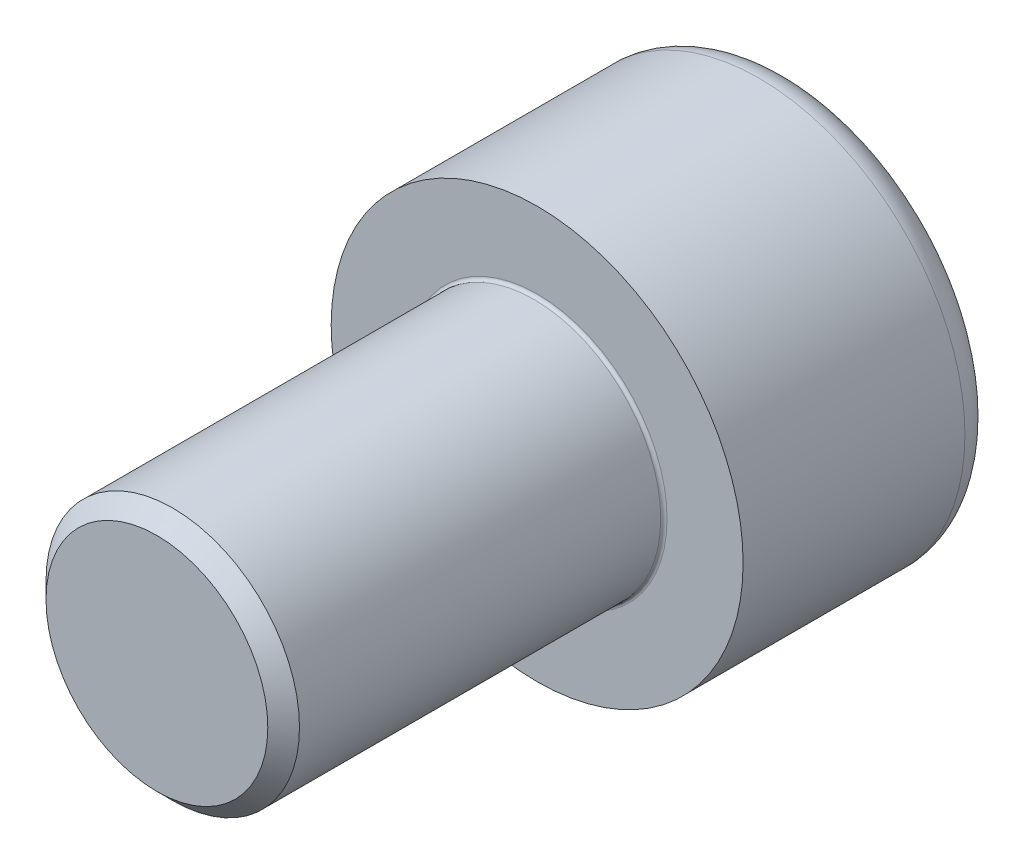
SolidWorks part; units mm, degrees
ref_plane "前视基准面" through (0, 0, 0) normal (0, 0, 1) x (1, 0, 0)
ref_plane "上视基准面" through (0, 0, 0) normal (0, 1, 0) x (1, 0, 0)
ref_plane "右视基准面" through (0, 0, 0) normal (1, 0, 0) x (0, 0, -1)
sketch "草图1" plane through (0, 0, 0) normal (0, 0, 1) x (1, 0, 0)
  circle A0 centre (0, 0) radius 6.5
  dimension "D1" = 13
extrude "凸台-拉伸1" add sketch "草图1" along normal blind 8 contours A0
sketch "草图2" plane through (0, 0, 8) normal (0, 0, 1) x (1, 0, 0)
  circle A0 centre (0, 0) radius 4
  dimension "D1" = 8
extrude "凸台-拉伸2" add sketch "草图2" along normal blind 12 contours A0
sketch "草图3" plane through (0, 0, 0) normal (0, 0, -1) x (-1, 0, 0)
  line L1 (1.7321, -3) -> (3.4641, 0)
  line L2 (3.4641, 0) -> (1.7321, 3)
  line L3 (1.7321, 3) -> (-1.7321, 3)
  line L4 (-1.7321, 3) -> (-3.4641, 0)
  line L5 (-3.4641, 0) -> (-1.7321, -3)
  line L6 (-1.7321, -3) -> (1.7321, -3)
  circle A0 centre (0, 0) radius 3 construction
  dimension "D1" = 6
extrude "切除-拉伸1" cut sketch "草图3" against normal blind 4
fillet "圆角1" radius 0.1 1 edges at (4, 0, 8)
chamfer "倒角1" distance 0.5 angle 45 1 edges at (4, 0, 20)
fillet "圆角2" radius 1 1 edges at (6.5, 0, 0)
